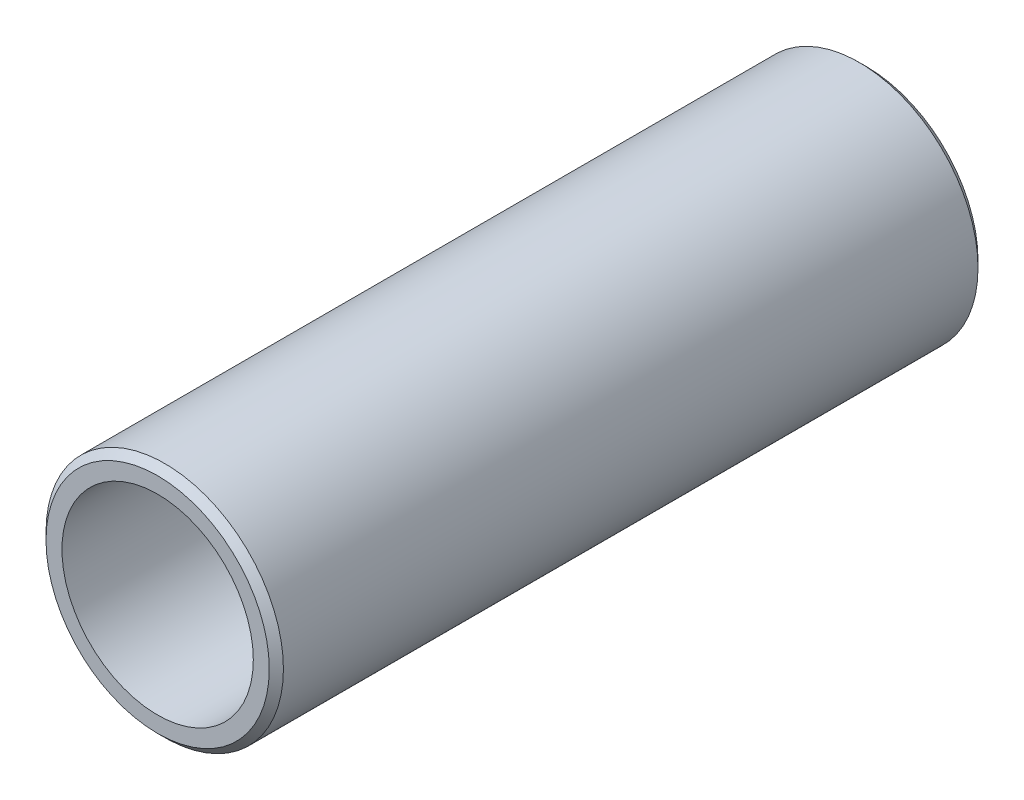
SolidWorks part; units mm, degrees
material "镀锌焊接钢管 Q215A"
ref_plane "前视基准面" through (0, 0, 0) normal (0, 0, 1) x (1, 0, 0)
ref_plane "上视基准面" through (0, 0, 0) normal (0, 1, 0) x (1, 0, 0)
ref_plane "右视基准面" through (0, 0, 0) normal (1, 0, 0) x (0, 0, -1)
sketch "草图1" plane through (0, 0, 0) normal (0, 0, 1) x (1, 0, 0)
  circle A0 centre (0, 0) radius 13.5
  circle A1 centre (0, 0) radius 16.75
  dimension "D2" = 33.5
  dimension "D1" = 3.25
extrude "凸台-拉伸1" add sketch "草图1" along normal blind 100
cosmetic thread "装饰螺纹线1" parameters "D1"=20, "D2"=30.291
cosmetic thread "装饰螺纹线3" parameters "D1"=20, "D2"=30.291
chamfer "倒角1" distance 1 angle 45 1 edges at (16.75, 0, 100)
chamfer "倒角2" distance 1 angle 45 1 edges at (16.75, 0, 0)
